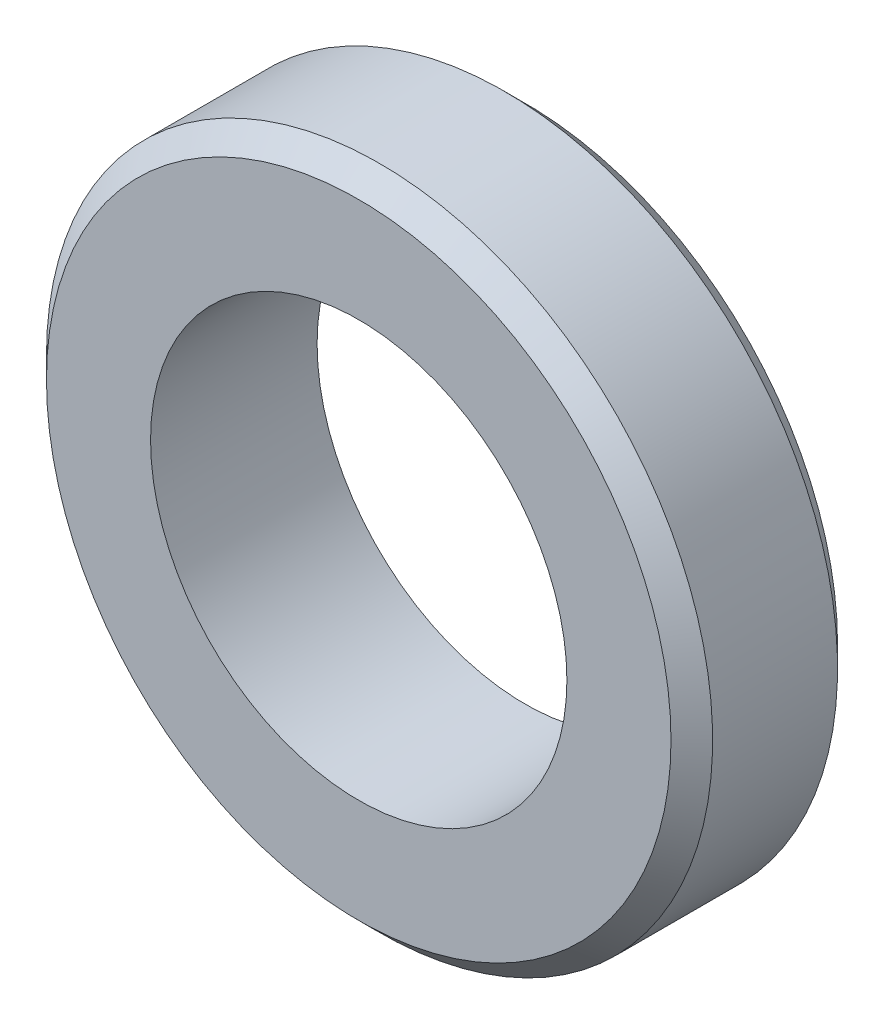
SolidWorks part; units mm, degrees
ref_plane "Front Plane" through (0, 0, 0) normal (0, 0, 1) x (1, 0, 0)
ref_plane "Top Plane" through (0, 0, 0) normal (0, 1, 0) x (1, 0, 0)
ref_plane "Right Plane" through (0, 0, 0) normal (1, 0, 0) x (0, 0, -1)
other "Configuration Table"
ref_plane "Plane1" through (0, 0, 0) normal (0, -1, 0) x (1, 0, 0)
sketch "Sketch1" plane through (0, 0, 0) normal (0, -1, 0) x (1, 0, 0)
  line L0 (5, 4) -> (5, 0)
  line L1 (5, 0) -> (7.5, 0)
  line L2 (7.5, 0) -> (8, 0.5)
  line L3 (8, 0.5) -> (8, 3.5)
  line L4 (8, 3.5) -> (7.5, 4)
  line L5 (7.5, 4) -> (5, 4)
  line L6 (0, 4) -> (0, 0) construction
revolve "Revolve1" add sketch "Sketch1" angle 360 about L6
